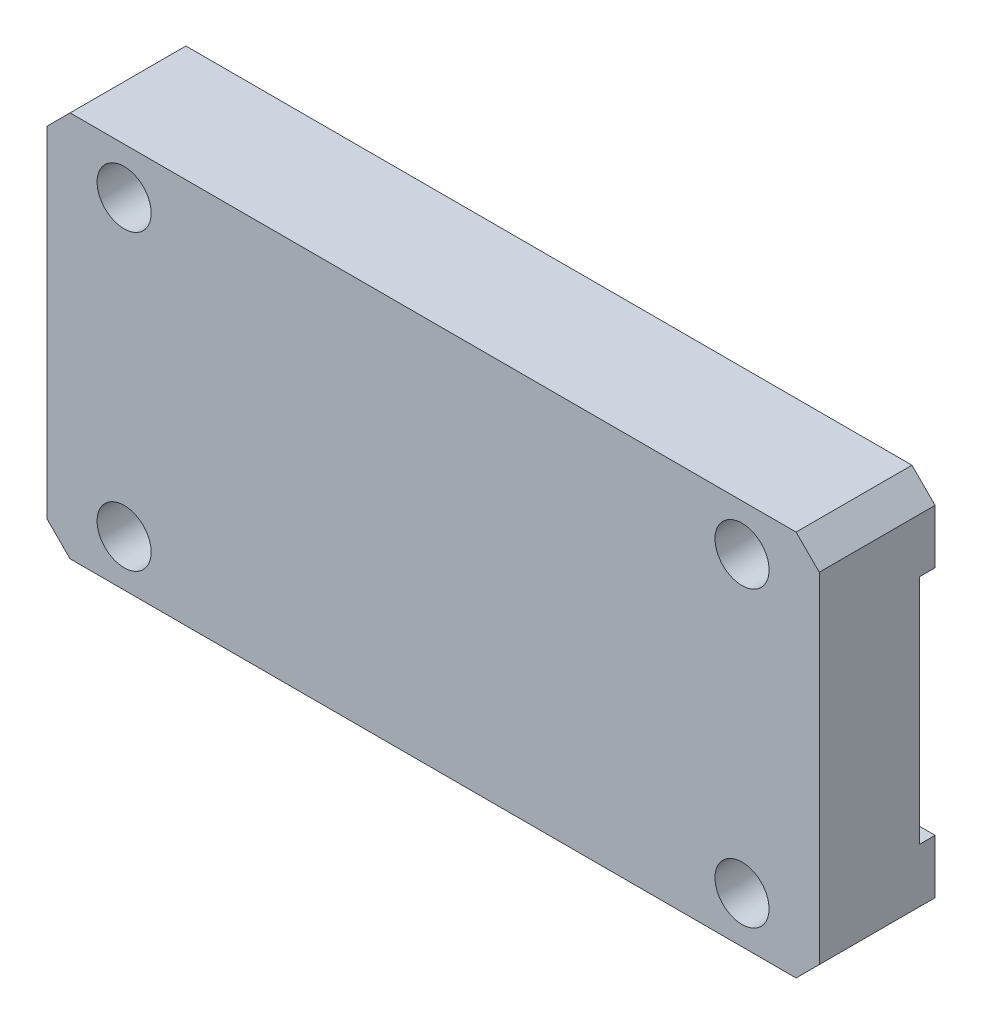
from build123d import *

# Parameters (mm, degrees)
SKETCH_1_W            = 100
SKETCH_1_H            = 50
EXTRUDE_1_DEPTH       = 15
HOLE_WIZARD_7_0_7_1_D = 7
CHAMFER_1_SIZE        = 3
SKETCH_6_W            = 2
SKETCH_6_H            = 30
CUT_EXTRUDE_1_DEPTH   = 113


with BuildPart() as part:
    # 草图1 → 凸台-拉伸1 (new body)
    with BuildSketch(Plane.XY):
        with Locations((50, 25)):
            Rectangle(SKETCH_1_W, SKETCH_1_H)
    extrude(amount=EXTRUDE_1_DEPTH)

    # Ø7.0 (7) 直径孔1 (through all)
    with Locations(Plane(origin=(0, 0, 0), x_dir=(-1, 0, 0), z_dir=(0, 0, -1))):
        with Locations((-10, 44), (-10, 6), (-90, 44), (-90, 6)):
            Hole(HOLE_WIZARD_7_0_7_1_D / 2)

    # 倒角1
    chamfer_1_edges = [part.edges().sort_by_distance(p)[0] for p in [
        (0, 50, 7.5),
        (100, 50, 7.5),
        (100, 0, 7.5),
        (0, 0, 7.5),
    ]]
    chamfer(chamfer_1_edges, length=CHAMFER_1_SIZE)

    # 草图6 → 切除-拉伸1 (cut)
    with BuildSketch(Plane.ZY):
        with Locations((1, 25)):
            Rectangle(SKETCH_6_W, SKETCH_6_H)
    extrude(amount=-CUT_EXTRUDE_1_DEPTH, mode=Mode.SUBTRACT)


solid = part.part
